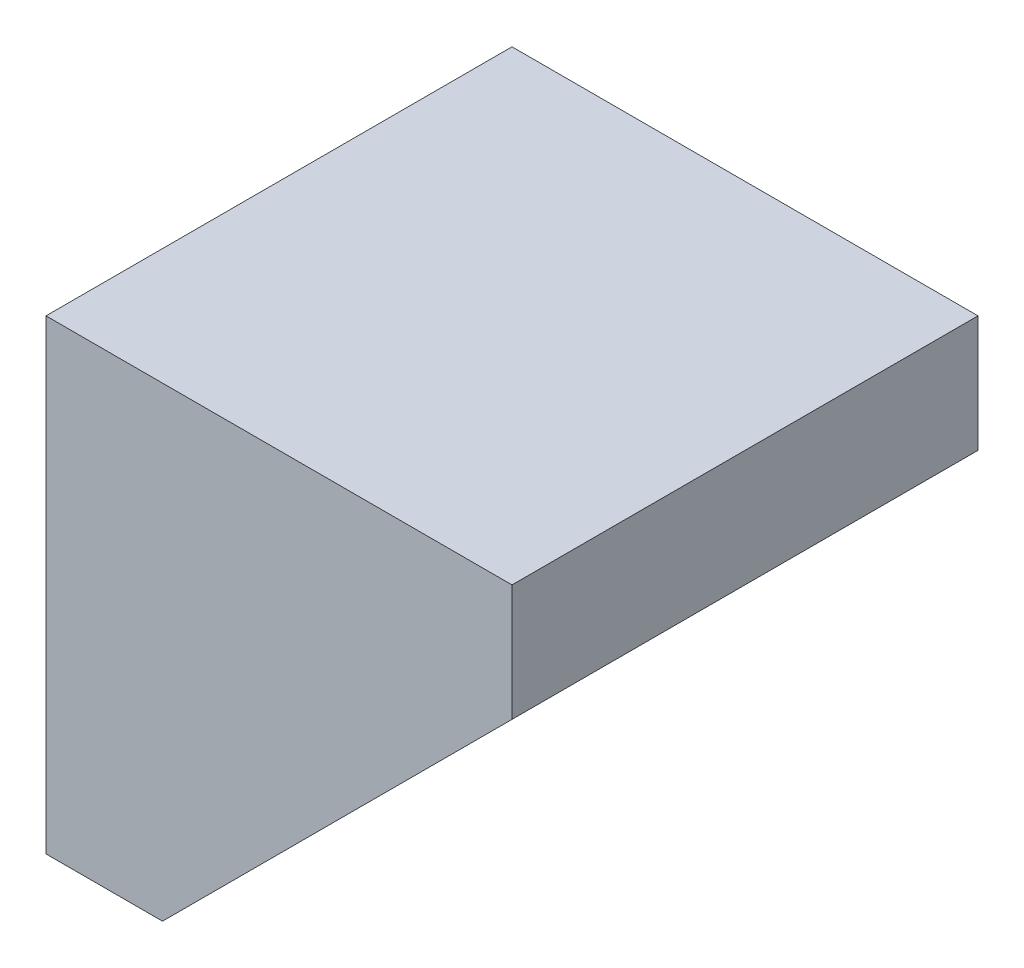
SolidWorks part; units mm, degrees
ref_plane "前视基准面" through (0, 0, 0) normal (0, 0, 1) x (1, 0, 0)
ref_plane "上视基准面" through (0, 0, 0) normal (0, 1, 0) x (1, 0, 0)
ref_plane "右视基准面" through (0, 0, 0) normal (1, 0, 0) x (0, 0, -1)
sketch "草图1" plane through (0, 0, 0) normal (1, 0, 0) x (0, 0, -1)
  line L1 (-40, 40) -> (40, 40)
  line L2 (-40, 40) -> (-40, -40)
  line L3 (-40, -40) -> (40, -40)
  line L4 (40, 40) -> (40, -40)
  line L5 (-40, 40) -> (40, -40) construction
  line L6 (-40, -40) -> (40, 40) construction
  point P0 (0, 0)
  dimension "D1" = 80
  dimension "D2" = 80
extrude "凸台-拉伸1" add sketch "草图1" along normal blind 80
hole_wizard "打孔尺寸(%根据)内六角圆柱头螺钉的类型1" positions "草图3" profile "草图4" counterbore size "M10" standard "GB" end condition through all
sketch "草图3" plane through (80, 0, 0) normal (1, 0, 0) x (0, 0, -1)
  line L0 (0, 0) -> (0, 23.7123) construction
  point P0 (-25, 0)
  point P2 (25, 0)
  dimension "D1" = 50
sketch "草图4" plane through (80, 0, 25) normal (0, 1, 0) x (0, 0, -1)
  line L0 (0, 0) -> (0, 80)
  line L1 (0, 80) -> (5.5, 80)
  line L3 (5.5, 80) -> (5.5, 50)
  line L4 (5.5, 50) -> (9, 50)
  line L5 (9, 50) -> (9, 0)
  line L7 (9, 0) -> (0, 0)
  line L11 (0, -6.35) -> (0, 107.95) construction
  dimension "通孔孔直径" = 11
  dimension "通孔孔深度" = 80
  dimension "柱形沉头孔直径" = 18
  dimension "柱形沉头孔深度" = 50
sketch "草图2" plane through (0, 0, 40) normal (0, 0, 1) x (1, 0, 0)
  line L0 (20, -40) -> (80, 20)
  line L1 (80, -40) -> (0, -40) construction
  line L3 (80, 20) -> (80, -40)
  line L4 (80, -40) -> (20, -40)
  line L6 (80, 40) -> (0, 40) construction
  dimension "D1" = 45
  dimension "D2" = 20
extrude "切除-拉伸1" cut sketch "草图2" against normal through all contours L0 L3 L4
